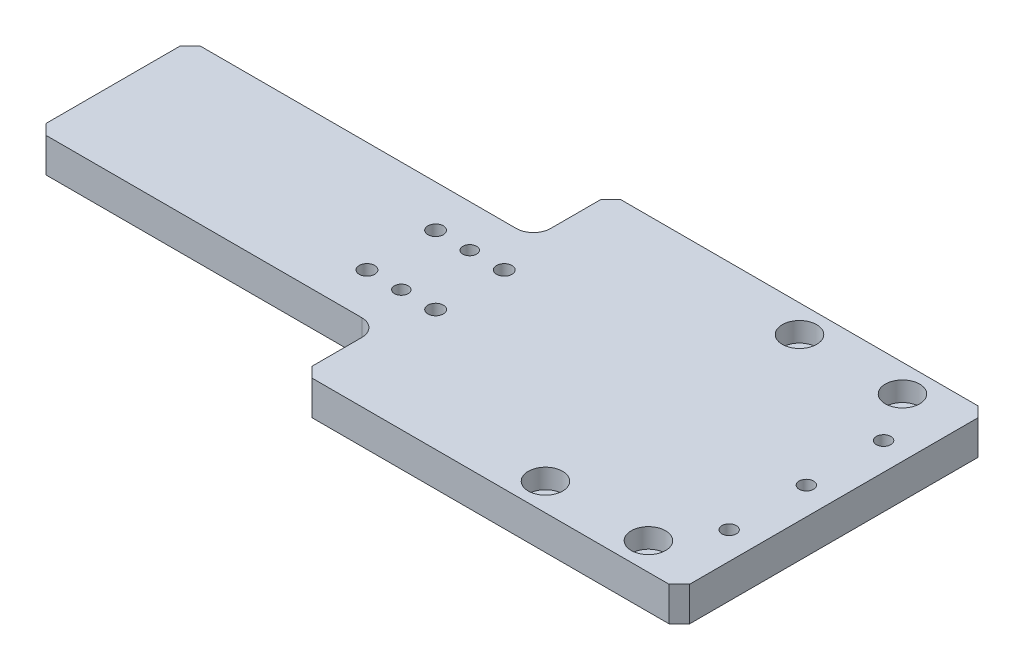
SolidWorks part; units mm, degrees
material "A6061 T6"
ref_plane "前视基准面" through (0, 0, 0) normal (0, 0, 1) x (1, 0, 0)
ref_plane "上视基准面" through (0, 0, 0) normal (0, 1, 0) x (1, 0, 0)
ref_plane "右视基准面" through (0, 0, 0) normal (1, 0, 0) x (0, 0, -1)
sketch "草图1" plane through (0, 0, 0) normal (0, 1, 0) x (1, 0, 0)
  line L1 (-105, 45) -> (105, 45)
  line L2 (-105, 45) -> (-105, -45)
  line L3 (-105, -45) -> (105, -45)
  line L4 (105, 45) -> (105, -45)
  line L5 (-105, 45) -> (105, -45) construction
  line L6 (-105, -45) -> (105, 45) construction
  point P0 (0, 0)
  dimension "D1" = 90
  dimension "D2" = 210
extrude "凸台-拉伸1" add sketch "草图1" along normal blind 10
chamfer "倒角1" distance 3 angle 45 4 edges at (-105, 5, -45) (105, 5, -45) (105, 5, 45) (-105, 5, 45)
hole_wizard "打孔尺寸(%根据)内六角圆柱头螺钉的类型2" positions "草图2" profile "草图3" counterbore size "M5" standard "GB"
sketch "草图2" plane through (0, 10, 0) normal (0, 1, 0) x (1, 0, 0)
  line L0 (-102, -45) -> (102, -45) construction
  line L1 (105, -42) -> (105, 42) construction
  point P0 (58, -37)
  point P3 (58, 37)
  point P6 (88, 37)
  point P9 (88, -37)
  dimension "D1" = 30
  dimension "D2" = 8
  dimension "D3" = 74
  dimension "D4" = 17
sketch "草图3" plane through (58, 10, 37) normal (1, 0, 0) x (0, 0, 1)
  line L0 (0, 0) -> (0, 11.7524)
  line L1 (0, 11.7524) -> (2.75, 10.1)
  line L2 (2.75, 10.1) -> (2.75, 5.7)
  line L3 (2.75, 5.7) -> (5, 5.7)
  line L4 (5, 5.7) -> (5, 0)
  line L5 (5, 0) -> (0, 0)
  line L10 (0, 11.7524) -> (-2.75, 10.1) construction
  line L11 (0, -6.35) -> (0, 107.95) construction
  dimension "孔直径" = 5.5
  dimension "孔深度" = 10.1
  dimension "柱形沉头孔直径" = 10
  dimension "柱形沉头孔深度" = 5.7
  dimension "导头角度" = 118
sketch "草图4" plane through (0, 10, 0) normal (0, 1, 0) x (1, 0, 0)
  line L0 (-105, 42) -> (-105, -42) construction
  line L1 (-105, -22.5) -> (-5, -22.5)
  line L2 (-105, -22.5) -> (-105, -45)
  line L3 (-105, -45) -> (-5, -45)
  line L4 (-5, -22.5) -> (-5, -45)
  line L5 (-102, -45) -> (102, -45) construction
  line L6 (102, 45) -> (-102, 45) construction
  line L7 (-105, 22.5) -> (-5, 22.5)
  line L8 (-105, 22.5) -> (-105, 45)
  line L9 (-105, 45) -> (-5, 45)
  line L10 (-5, 22.5) -> (-5, 45)
  dimension "D1" = 45
  dimension "D2" = 100
extrude "切除-拉伸1" cut sketch "草图4" against normal blind 20
chamfer "倒角2" distance 3 angle 45 4 edges at (-5, 5, -45) (-5, 5, 45) (-105, 5, -22.5) (-105, 5, 22.5)
fillet "圆角1" radius 5 2 edges at (-5, 5, -22.5) (-5, 5, 22.5)
hole_wizard "打孔尺寸(%根据)内六角圆柱头螺钉的类型0" positions "草图5" profile "草图6" counterbore size "M4" standard "GB"
sketch "草图5" plane through (0, 0, 0) normal (0, -1, 0) x (-1, 0, 0)
  point P0 (21.3, 10.3)
  point P3 (21.3, -9.7)
  point P6 (1.3, 10.3)
  point P9 (1.3, -9.7)
sketch "草图6" plane through (-21.3, 0, -10.3) normal (1, 0, 0) x (0, 0, -1)
  line L0 (0, 0) -> (0, 26.3519)
  line L1 (0, 26.3519) -> (2.25, 25)
  line L2 (2.25, 25) -> (2.25, 4.6)
  line L3 (2.25, 4.6) -> (4, 4.6)
  line L4 (4, 4.6) -> (4, 0)
  line L5 (4, 0) -> (0, 0)
  line L10 (0, 26.3519) -> (-2.25, 25) construction
  line L11 (0, -6.35) -> (0, 107.95) construction
  dimension "孔直径" = 4.5
  dimension "孔深度" = 25
  dimension "柱形沉头孔直径" = 8
  dimension "柱形沉头孔深度" = 4.6
  dimension "导头角度" = 118
hole_wizard "大小mm 暗销孔0" positions "草图7" profile "草图8" hole size "Ø4.0" standard "GB"
sketch "草图7" plane through (0, 0, 0) normal (0, -1, 0) x (-1, 0, 0)
  point P0 (11.3, -9.7)
  point P3 (11.3, 10.2317)
sketch "草图8" plane through (-11.3, 0, 9.7) normal (1, 0, 0) x (0, 0, -1)
  line L0 (0, 0) -> (0, 26.2017)
  line L1 (0, 26.2017) -> (2, 25)
  line L2 (2, 25) -> (2, 0)
  line L5 (2, 0) -> (0, 0)
  line L10 (0, 26.2017) -> (-2, 25) construction
  line L11 (0, -6.35) -> (0, 107.95) construction
  dimension "孔直径" = 4
  dimension "孔深度" = 25
  dimension "导头角度" = 118
hole_wizard "M5 螺纹孔1" positions "草图9" profile "草图10" tap size "M5" standard "GB"
sketch "草图9" plane through (0, 10, 0) normal (0, 1, 0) x (1, 0, 0)
  point P0 (97, -22.5)
  point P3 (97, 0)
  point P6 (97, 22.5)
sketch "草图10" plane through (97, 10, 22.5) normal (1, 0, 0) x (0, 0, 1)
  line L0 (0, 0) -> (0, 13.6618)
  line L1 (0, 13.6618) -> (2.1, 12.4)
  line L2 (2.1, 12.4) -> (2.1, 0)
  line L5 (2.1, 0) -> (0, 0)
  line L10 (0, 13.6618) -> (-2.1, 12.4) construction
  line L11 (0, -6.35) -> (0, 107.95) construction
  dimension "螺纹孔钻头直径" = 4.2
  dimension "螺纹孔钻头深度" = 12.4
  dimension "导头角度" = 118
cosmetic thread "孔螺蚊线1"
cosmetic thread "孔螺蚊线2"
cosmetic thread "孔螺蚊线3"
